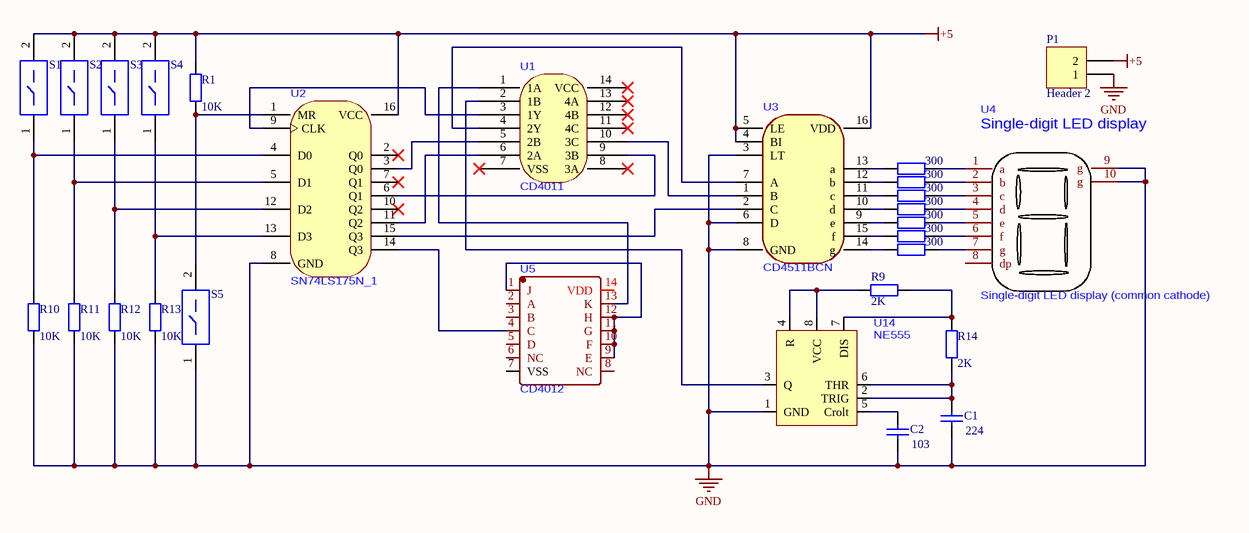
[diagram p0: MISC80628-3.SchDoc]
# Altium project MISC80628-21.PrjPcb
1 sheet, 28 parts. Net scope: global (net labels, ports and power ports of the same name join across sheets).
Board file: MISC80628.PcbDoc

## Sheet MISC80628-3.SchDoc
size A4

### Parts
C1  value 224  [RAD-0.3]  (hidden comment: Cap)
C2  value 103  [RAD-0.3]  (hidden comment: Cap)
P1  Header 2  [HDR1X2]
R1  value 10K  [AXIAL-0.4]  (hidden comment: Res2)
R2  value 300  [AXIAL-0.4]  (hidden comment: Res2)
R3  value 300  [AXIAL-0.4]  (hidden comment: Res2)
R4  value 300  [AXIAL-0.4]  (hidden comment: Res2)
R5  value 300  [AXIAL-0.4]  (hidden comment: Res2)
R6  value 300  [AXIAL-0.4]  (hidden comment: Res2)
R7  value 300  [AXIAL-0.4]  (hidden comment: Res2)
R8  value 300  [AXIAL-0.4]  (hidden comment: Res2)
R9  value 2K  [AXIAL-0.4]  (hidden comment: Res2)
R10  value 10K  [AXIAL-0.4]  (hidden comment: Res2)
R11  value 10K  [AXIAL-0.4]  (hidden comment: Res2)
R12  value 10K  [AXIAL-0.4]  (hidden comment: Res2)
R13  value 10K  [AXIAL-0.4]  (hidden comment: Res2)
R14  value 2K  [AXIAL-0.4]  (hidden comment: Res2)
S1  SW1-DIP2  [DIP-1P]  (value not drawn)
S2  SW1-DIP2  [DIP-1P]  (value not drawn)
S3  SW1-DIP2  [DIP-1P]  (value not drawn)
S4  SW1-DIP2  [DIP-1P]  (value not drawn)
S5  SW1-DIP2  [DIP-1P]  (value not drawn)
U1  CD4011  [CD4011]
U2  SN74LS175N_1  [N016]
U3  CD4511BCN  [CD4511BCN]
U4  Single-digit LED display (common cathode)  [PCBComponent_1]
U5  CD4012  [DIP14]
U14  NE555  [DIP-8-NE555]

### Nets
+5: P1.2 R1.2 S1.2 S2.2 S3.2 S4.2 U2.16(VCC) U3.4(BI) U3.5(LE) U3.16(VDD)
GND: C1.1 C2.1 P1.1 R10.1 R11.1 R12.1 R13.1 S5.1(A1) U2.8(GND) U3.3(LT) U3.6(D) U3.8(GND) U4.9(g) U4.10(g) U14.1(GND)
NetC1_2: C1.2 R14.1 U14.2(TRIG) U14.6(THR)
NetC2_2: C2.2 U14.5(Crolt)
NetR1_1: R1.1 S5.2 U2.1(MR)
NetR2_1: R2.1 U4.1(a)
NetR2_2: R2.2 U3.13(a)
NetR3_1: R3.1 U4.2(b)
NetR3_2: R3.2 U3.12(b)
NetR4_1: R4.1 U4.3(c)
NetR4_2: R4.2 U3.11(c)
NetR5_1: R5.1 U4.4(d)
NetR5_2: R5.2 U3.10(d)
NetR6_1: R6.1 U4.5(e)
NetR6_2: R6.2 U3.9(e)
NetR7_1: R7.1 U4.6(f)
NetR7_2: R7.2 U3.15(f)
NetR8_1: R8.1 U4.7(g)
NetR8_2: R8.2 U3.14(g)
NetR9_1: R9.1 R14.2 U14.7(DIS)
NetR9_2: R9.2 U14.4(R) U14.8(VCC)
NetR10_2: R10.2 S1.1(A1) U2.4(D0)
NetR11_2: R11.2 S2.1(A1) U2.5(D1)
NetR12_2: R12.2 S3.1(A1) U2.12(D2)
NetR13_2: R13.2 S4.1(A1) U2.13(D3)
NetU1_1: U1.1(1A) U5.13(K)
NetU1_2: U1.2(1B) U14.3(Q)
NetU1_3: U1.3(1Y) U2.9(CLK)
NetU1_4: U1.4(2Y) U3.7(A)
NetU1_5: U1.5(2B) U2.3(Q0)
NetU1_6: U1.6(2A) U2.11(Q2)
NetU1_9: U1.9(3B) U2.6(Q1)
NetU1_10: U1.10(3C) U3.1(B)
NetU2_14: U2.14(Q3) U5.4(C)
NetU2_15: U2.15(Q3) U3.2(C)
NetU5_1: U5.1(J) U5.9(E) U5.10(F) U5.11(G) U5.12(H)

Not connected (* = marked no-connect by the designer): U1 7(VSS)* 8(3A)* 11(4C)* 12(4B)* 13(4A)* 14(VCC)*; U2 2(Q0)* 7(Q1)* 10(Q2)*; U4 8(dp); U5 2(A) 3(B) 5(D) 6(NC) 7(VSS) 8(NC) 14(VDD)

### Library data of the parts
C1 C2 = Cap: Capacitor; Published: 8-Jun-2000; LatestRevisionDate: 17-Jul-2002; LatestRevisionNote: Re-released for DXP Platform.; PackageReference: RAD-0.3; PackageDescription: Radial Cap, Thru-Hole; 2 Leads; 0.3 in Pin Spacing; Publisher: Altium Limited
P1 = Header 2: Header, 2-Pin; LatestRevisionDate: 17-Jul-2002; LatestRevisionNote: Re-released for DXP Platform.; Publisher: Altium Limited
R1-R14 = Res2: Resistor; Published: 8-Jun-2000; LatestRevisionDate: 17-Jul-2002; LatestRevisionNote: Re-released for DXP Platform.; PackageReference: AXIAL-0.4; PackageDescription: Axial Device, Thru-Hole; 2 Leads; 0.4 in Pin Spacing; Publisher: Altium Limited
U4 = 一位数码管（共阴极）
U5 = CD4012BM
U14 = NE555 (2)